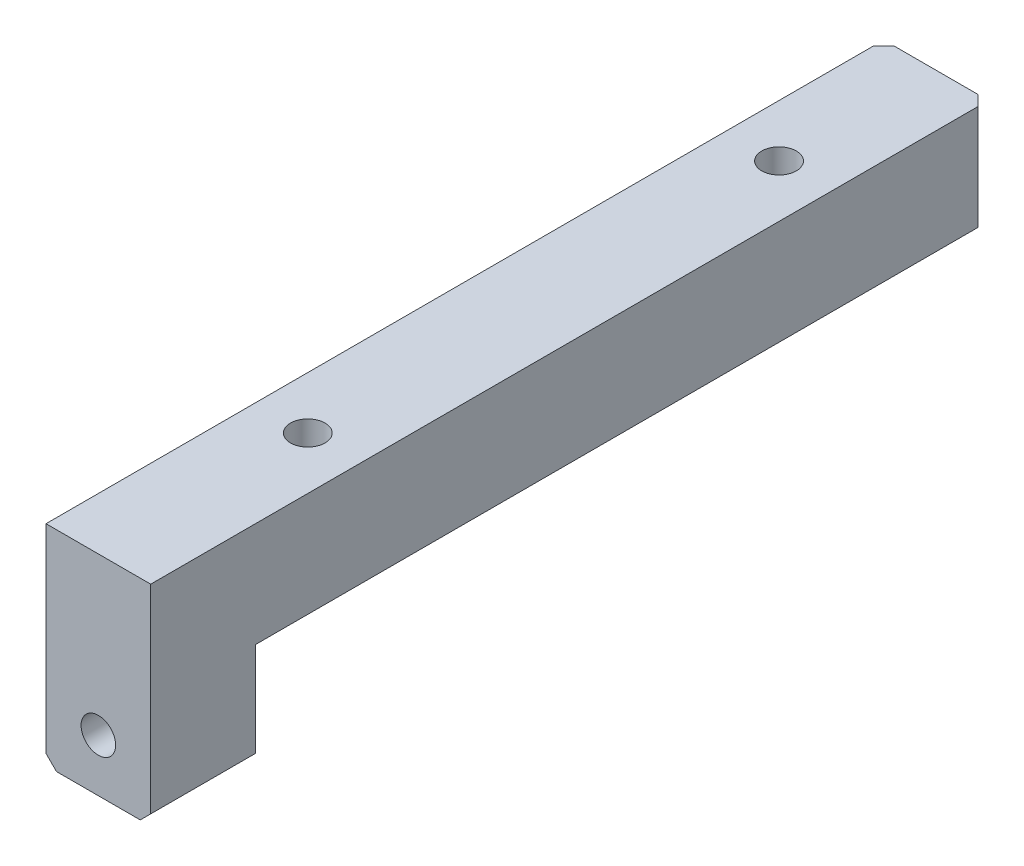
from build123d import *

# Parameters (mm, degrees)
SKETCH1_W             = 80
SKETCH1_H             = 20
BOSS_EXTRUDE1_DEPTH   = 10
SKETCH3_W             = 70
SKETCH3_H             = 10
CUT_EXTRUDE1_DEPTH    = 43.426406871
M4_TAPPED_HOLE2_D     = 3.3
M4_TAPPED_HOLE2_DEPTH = 10.1
M4_TAPPED_HOLE2_TIP   = 0.991420021
CHAMFER1_SIZE         = 1
M4_TAPPED_HOLE1_D     = 3.3
M4_TAPPED_HOLE1_DEPTH = 10.1
M4_TAPPED_HOLE1_TIP   = 0.991420021


with BuildPart() as part:
    # Sketch1 → Boss-Extrude1 (new body)
    with BuildSketch(Plane(origin=(0, 0, 0), x_dir=(0, 0, -1), z_dir=(1, 0, 0))):
        Rectangle(SKETCH1_W, SKETCH1_H)
    extrude(amount=BOSS_EXTRUDE1_DEPTH)

    # Sketch3 → Cut-Extrude1 (cut, through all)
    with BuildSketch(Plane.ZY):
        with Locations((-5, -5)):
            Rectangle(SKETCH3_W, SKETCH3_H)
    extrude(amount=-CUT_EXTRUDE1_DEPTH, mode=Mode.SUBTRACT)

    # M4 Tapped Hole2
    with Locations(Plane(origin=(0, 0, 30), x_dir=(-1, 0, 0), z_dir=(0, 0, -1))):
        with Locations((-5, -5)):
            Hole(M4_TAPPED_HOLE2_D / 2, depth=M4_TAPPED_HOLE2_DEPTH)
            with Locations((0, 0, -(M4_TAPPED_HOLE2_DEPTH + M4_TAPPED_HOLE2_TIP / 2))):  # 118° drill point
                Cone(0, M4_TAPPED_HOLE2_D / 2, M4_TAPPED_HOLE2_TIP, mode=Mode.SUBTRACT)

    # Chamfer1
    chamfer1_edges = [part.edges().sort_by_distance(p)[0] for p in [
        (0, 5, -40),
        (10, 5, -40),
        (10, -10, 35),
        (0, -10, 35),
    ]]
    chamfer(chamfer1_edges, length=CHAMFER1_SIZE)

    # M4 Tapped Hole1
    with Locations(Plane(origin=(0, 10, 0), x_dir=(1, 0, 0), z_dir=(0, 1, 0))):
        with Locations((5, 25), (5, -20)):
            Hole(M4_TAPPED_HOLE1_D / 2, depth=M4_TAPPED_HOLE1_DEPTH)
            with Locations((0, 0, -(M4_TAPPED_HOLE1_DEPTH + M4_TAPPED_HOLE1_TIP / 2))):  # 118° drill point
                Cone(0, M4_TAPPED_HOLE1_D / 2, M4_TAPPED_HOLE1_TIP, mode=Mode.SUBTRACT)


solid = part.part
